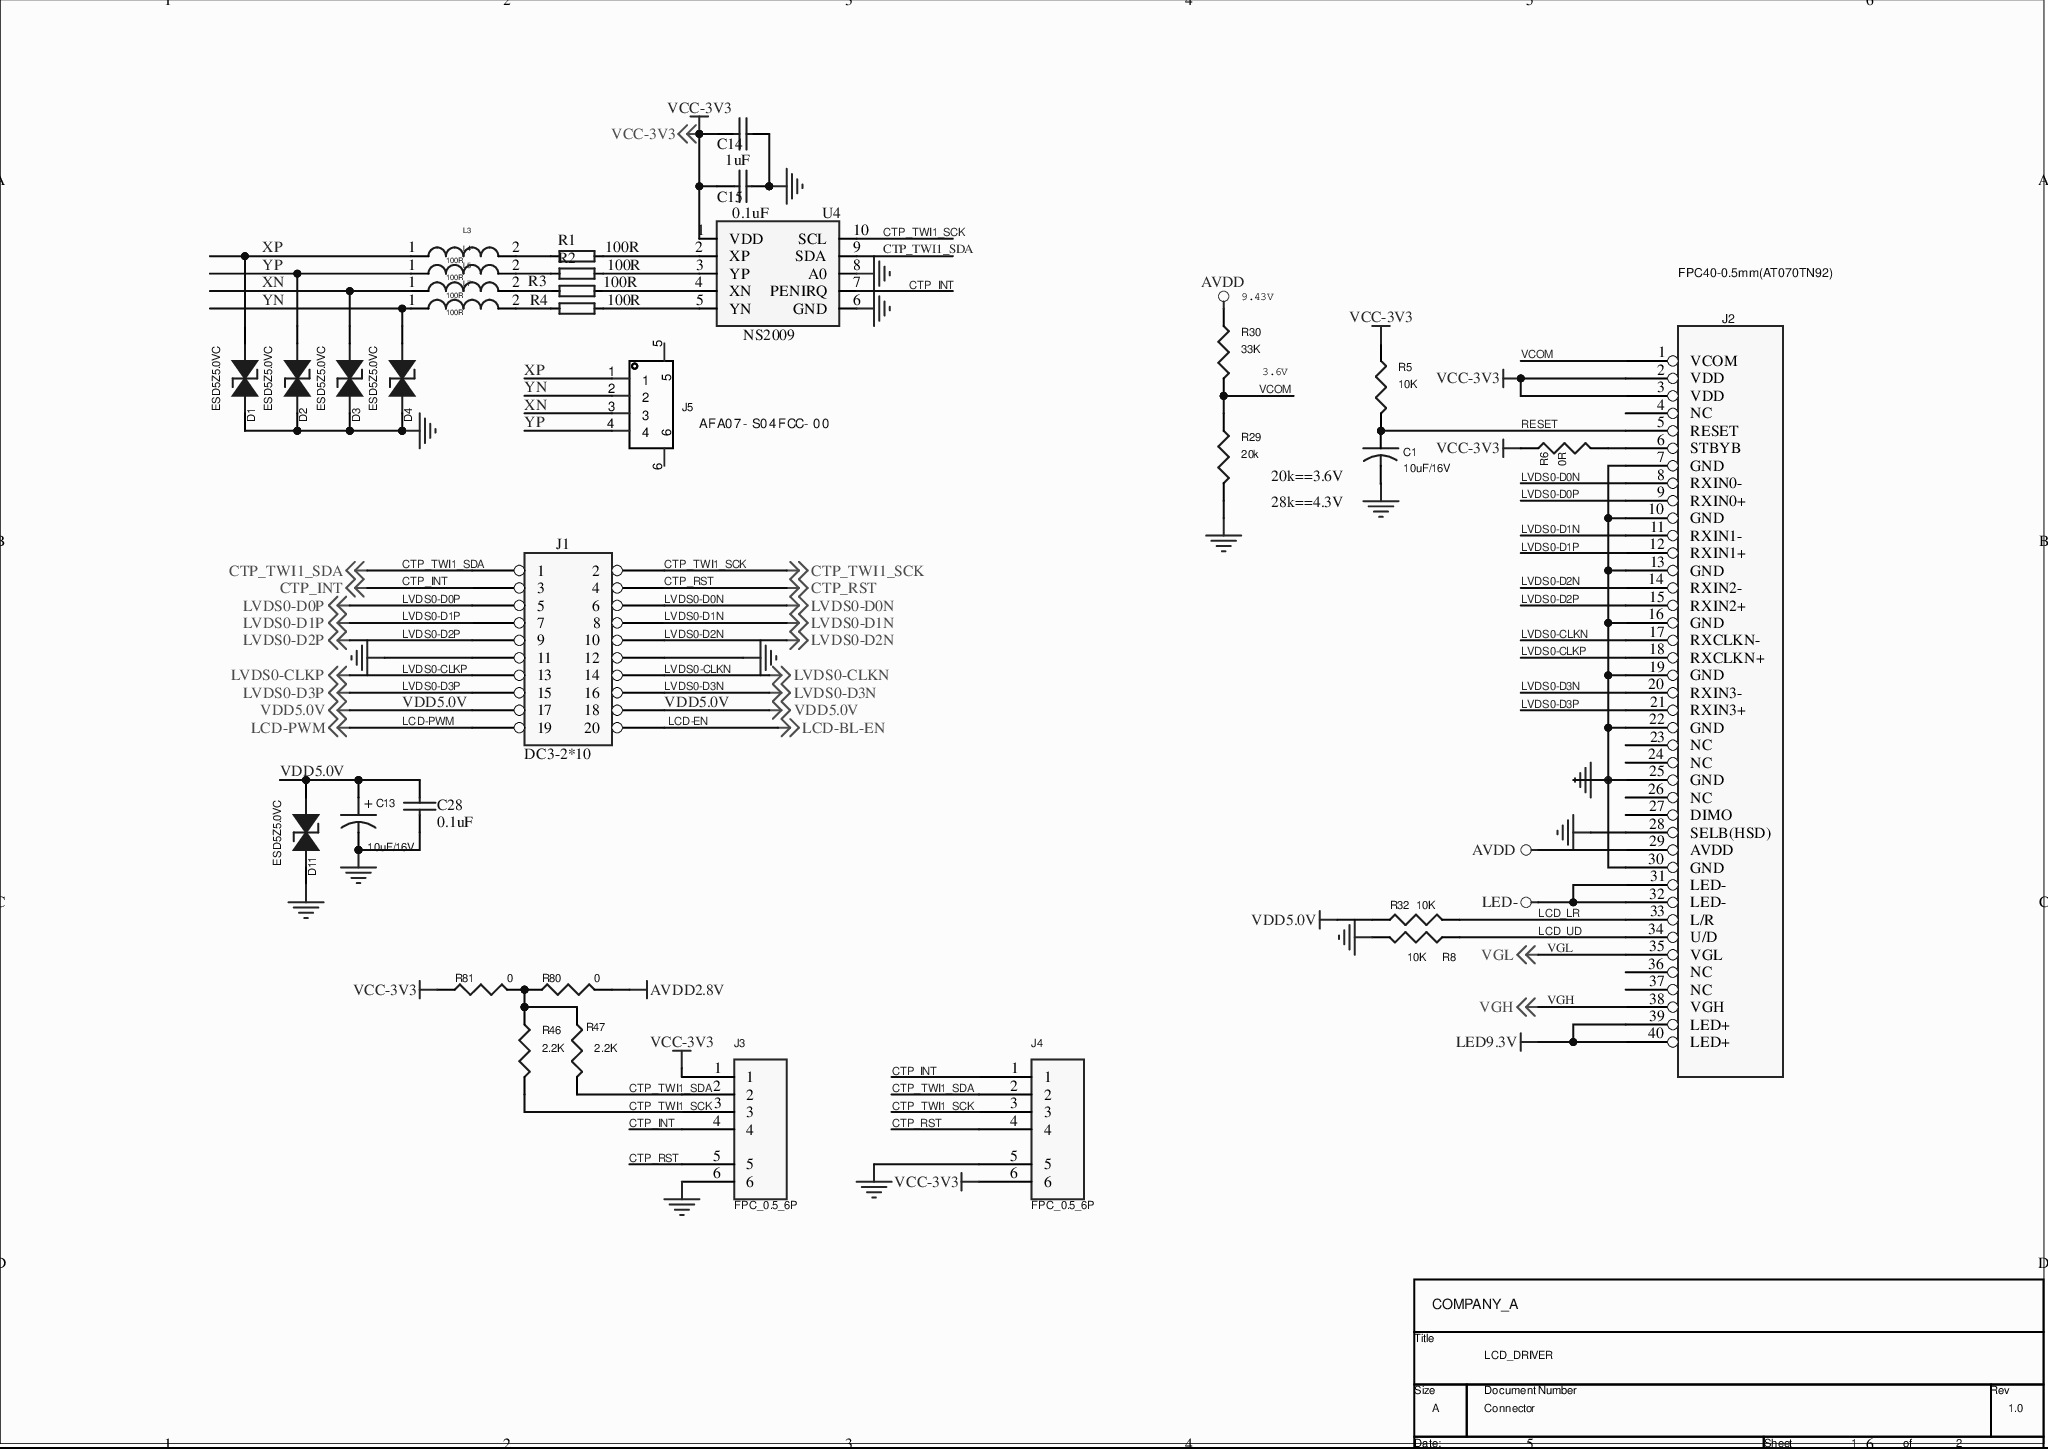
[diagram p0: MISC82162-14.SchDoc]
# Altium project MISC82162-6.PrjPcb
2 sheets, 91 parts. Net scope: global (net labels, ports and power ports of the same name join across sheets).
Board file: MISC82162.PcbDoc
Sheets:
  MISC82162-14.SchDoc
  MISC82162-10.SchDoc

## Sheet MISC82162-14.SchDoc
size 297 x 209 mm

### Parts
*  Page Count: 2  Page Number: 1  Page Size: A  OrgName: COMPANY_A  Title: LCD_DRIVER  RevCode: 1.0  Doc: Connector  (hidden comment: TitleBlock1)  (graphical)
C1  10uF/16V  [0603C]
C13  10uF/16V  [0805C]
C14  1uF  [0603C]
C15  0.1uF  [0603C]
C28  0.1uF  [0603C]
D1  ESD5Z5.0VC  [SOD-523]
D2  ESD5Z5.0VC  [SOD-523]
D3  ESD5Z5.0VC  [SOD-523]
D4  ESD5Z5.0VC  [SOD-523]
D11  ESD5Z5.0VC  [SOD-523]
J1  DC3-2*10  [DC3-2.0-2*10P]
J2  FPC40-0.5mm(AT070TN92)  [FPC40-0.5MM-UP]
J3  FPC_0.5_6P  [FPC_0.5_6P_UP]
J4  FPC_0.5_6P  [FPC_0.5_6P_DOWN]
J5  AFA07-S04FCC-00  [FPC-SMD-1mm4P-RTP]
L3  100R  [0603R]
L4  100R  [0603R]
L5  100R  [0603R]
L7  100R  [0603R]
R1  100R  [0603R]
R2  100R  [0603R]
R3  100R  [0603R]
R4  100R  [0603R]
R5  10K  [0603R]
R6  0R  [0603R]
R8  10K  [0603R]
R29  20k  [0603R]
R30  33K  [0603R]
R32  10K  [0603R]
R46  2.2K  [0603R]
R47  2.2K  [0603R]
R80  0  [0603R]
R81  0  [0603R]
U4  NS2009  [MSOP-10]

### Nets
AVDD: J2.29(AVDD) R30.1
AVDD2.8V: R80.2
GND: C1.2 C13.2 C14.2 C15.2 C28.1 D1.2(CATHODE) D2.2(CATHODE) D3.2(CATHODE) D4.2(CATHODE) D11.2(CATHODE) J1.11 J1.12 J2.7(GND) J2.10(GND) J2.13(GND) J2.16(GND) J2.19(GND) J2.22(GND) J2.25(GND) J2.28(SELB(HSD)) J2.30(GND) J3.6 J4.5 R8.2 R29.2 U4.6(GND) U4.8(A0)
LED9.3V: J2.39(LED+) J2.40(LED+)
LED-: J2.31(LED-) J2.32(LED-)
VCC-3V3: C14.1 C15.1 J2.2(VDD) J2.3(VDD) J3.1 J4.6 R5.1 R6.1 R81.1 U4.1(VDD) ; off-sheet VCC-3V3
VDD5.0V: C13.1 C28.2 D11.1(ANODE) J1.17 J1.18 R32.1 ; off-sheet VDD5.0V
VGH: J2.38(VGH) ; off-sheet VGH
VGL: J2.35(VGL) ; off-sheet VGL
CTP_INT: J1.3 J3.4 J4.1 U4.7(PENIRQ) ; off-sheet CTP_INT
CTP_RST: J1.4 J3.5 J4.4 ; off-sheet CTP_RST
CTP_TWI1_SCK: J1.2 J3.3 J4.3 R46.2 U4.10(SCL) ; off-sheet CTP_TWI1_SCK
CTP_TWI1_SDA: J1.1 J3.2 J4.2 R47.2 U4.9(SDA) ; off-sheet CTP_TWI1_SDA
LCD-BL-EN: J1.20 ; off-sheet LCD-BL-EN  [also labelled LCD-EN]
LCD-PWM: J1.19 ; off-sheet LCD-PWM
LCD_LR: J2.33(L/R) R32.2
LCD_UD: J2.34(U/D) R8.1
LVDS0-CLKN: J1.14 J2.17(RXCLKN-) ; off-sheet LVDS0-CLKN
LVDS0-CLKP: J1.13 J2.18(RXCLKN+) ; off-sheet LVDS0-CLKP
LVDS0-D0N: J1.6 J2.8(RXIN0-) ; off-sheet LVDS0-D0N
LVDS0-D0P: J1.5 J2.9(RXIN0+) ; off-sheet LVDS0-D0P
LVDS0-D1N: J1.8 J2.11(RXIN1-) ; off-sheet LVDS0-D1N
LVDS0-D1P: J1.7 J2.12(RXIN1+) ; off-sheet LVDS0-D1P
LVDS0-D2N: J1.10 J2.14(RXIN2-) ; off-sheet LVDS0-D2N
LVDS0-D2P: J1.9 J2.15(RXIN2+) ; off-sheet LVDS0-D2P
LVDS0-D3N: J1.16 J2.20(RXIN3-) ; off-sheet LVDS0-D3N
LVDS0-D3P: J1.15 J2.21(RXIN3+) ; off-sheet LVDS0-D3P
RESET: C1.1 J2.5(RESET) R5.2
VCOM: J2.1(VCOM) R29.1 R30.2
XN: D3.1(ANODE) J5.3 L5.1
XP: D1.1(ANODE) J5.1 L3.1
YN: D4.1(ANODE) J5.2 L7.1
YP: D2.1(ANODE) J5.4 L4.1
NetJ2_6: J2.6(STBYB) R6.2
NetL3_2: L3.2 R1.1
NetL4_2: L4.2 R2.1
NetL5_2: L5.2 R3.1
NetL7_2: L7.2 R4.1
NetR1_2: R1.2 U4.2(XP)
NetR2_2: R2.2 U4.3(YP)
NetR3_2: R3.2 U4.4(XN)
NetR4_2: R4.2 U4.5(YN)
NetR46_1: R46.1 R47.1 R80.1 R81.2

Not connected (* = marked no-connect by the designer): J2 4(NC) 23(NC) 24(NC) 26(NC) 27(DIMO) 36(NC) 37(NC); J5 5 6

### Notes on the sheet
- (near R30) 9.43V
- (near R30) 3.6V
- 20k==3.6V
- 28k==4.3V

### Library data of the parts
C1 = C
C13 = CAP POL
C14 C15 C28 = CAP: Capacitor
D1-D4 D11 = 1_1.5KE100A: 1ST PART DESCRIPTION: WILL ESD9B5V Bidirection ESD Protection
J2 = HEADER 20X2_3: Populate: YES
J3 J4 = connet_0
J5 = AFC07-S04ECC-00: Manufacturer: JS(钜硕电子); Symbol: FPC 0.5MM 4P Pull type H2.0mm Pick up; Add into BOM: yes; Pitch: 0.5mm; Number of Contacts: 4; Locking Feature: Drawer type; FFC, FCB Thickness: 0.3mm; Name: AFC07-S04ECC-00; Device: AFC07-S04ECC-00; LCSC Part Name: 0.5mm P数:4 抽屉式 上接; Supplier Part: C11082; Manufacturer Part: AFC07-S04ECC-00; Supplier Footprint: SMD,P=0.5mm; JLCPCB Part Class: Extended Part; Supplier: LCSC; Convert to PCB: yes; Mounting Type: Horizontal mount; Contact Type: Top entry; Height Above Board: 2mm
L3-L5 L7 = INDUCTOR
R1 R2 R4 = RES2
R3 = RES2: Designator: R?
R5 R6 R8 R29 R30 R32 R46 R47 R80 R81 = R
* = TitleBlock1: Page Create Date: March  8, 1995

## Sheet MISC82162-10.SchDoc
size A4
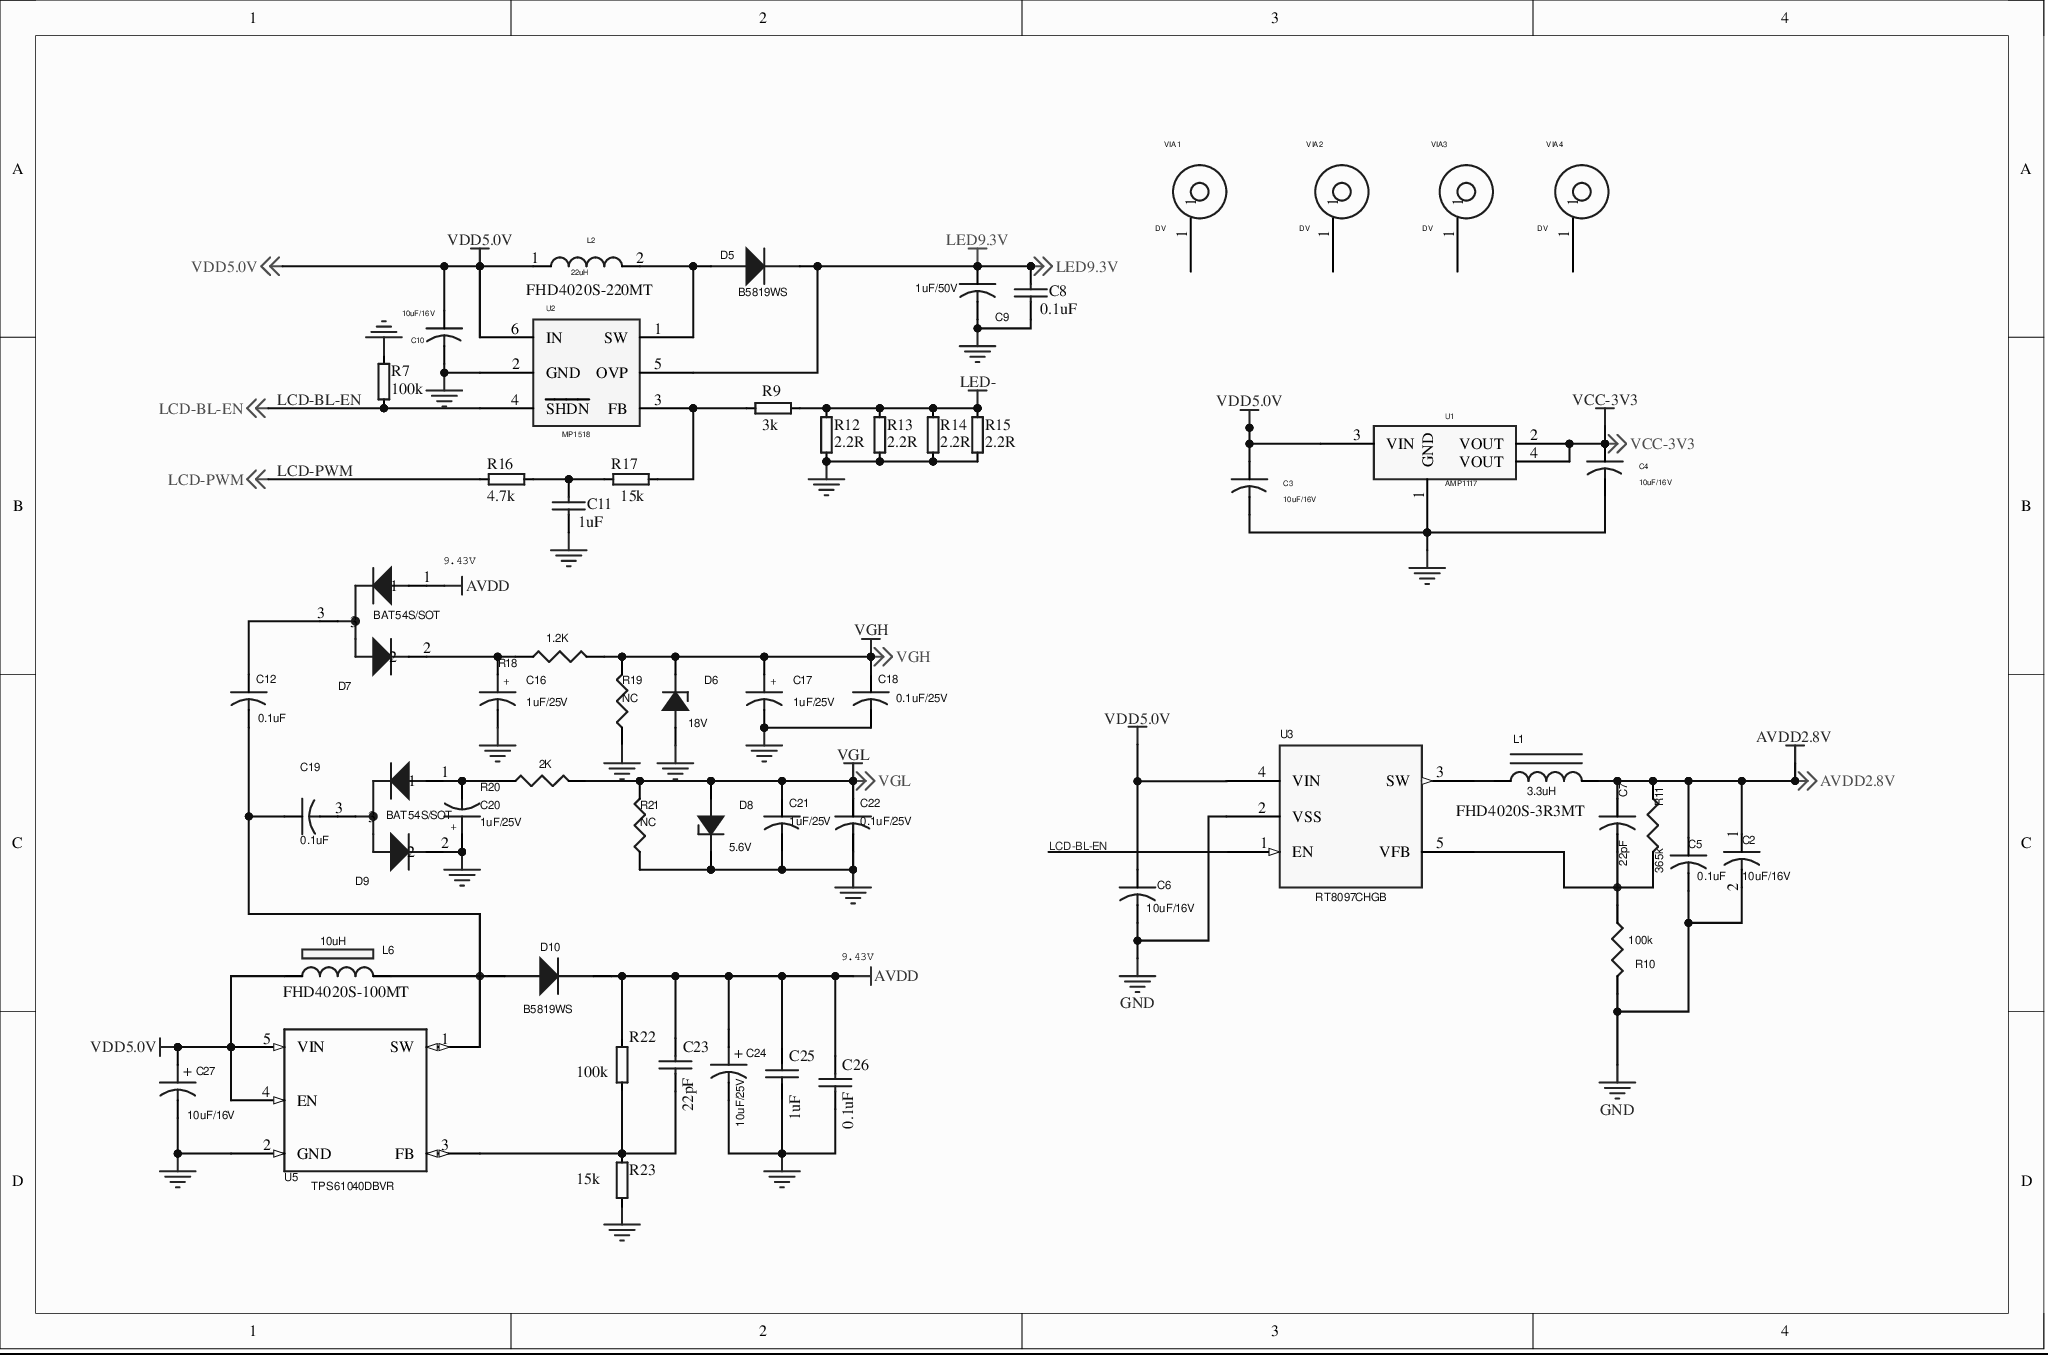
[diagram p1: MISC82162-10.SchDoc]

### Parts
C2  10uF/16V  [0805C]
C3  10uF/16V  [0805C]
C4  10uF/16V  [0805C]
C5  0.1uF  [0603C]
C6  10uF/16V  [0805C]
C7  22pF  [0603C]
C8  0.1uF  [0603C]
C9  1uF/50V  [0603C]
C10  10uF/16V  [0805C]
C11  1uF  [0603C]
C12  0.1uF  [0603C]
C16  1uF/25V  [0805C]
C17  1uF/25V  [0805C]
C18  0.1uF/25V  [0603C]
C19  0.1uF  [0603C]
C20  1uF/25V  [0805C]
C21  1uF/25V  [0603C]
C22  0.1uF/25V  [0603C]
C23  22pF  [0603C]
C24  10uF/25V  [0805C]
C25  1uF  [0603C]
C26  0.1uF  [0603C]
C27  10uF/16V  [0805C]
D5  B5819WS  [SOD-123]
D6  18V  [SOD-123]
D7  BAT54S/SOT  [SOT23]
D8  5.6V  [SOD-123]
D9  BAT54S/SOT  [SOT23]
D10  B5819WS  [SOD-123]
L1  3.3uH  [L-SMD-4*4*1.2]
L2  22uH  [L-SMD-4*4*1.2]
L6  10uH  [L-SMD-4*4*1.2]
R7  100k  [0603R]
R9  3k  [0603R]
R10  100k  [0603C]
R11  365k  [0603R]
R12  2.2R  [0805R]
R13  2.2R  [0805R]
R14  2.2R  [0805R]
R15  2.2R  [0805R]
R16  4.7k  [0603R]
R17  15k  [0603R]
R18  1.2K  [0603R]
R19  NC  [0603R]
R20  2K  [0603R]
R21  NC  [0603R]
R22  100k  [0603R]
R23  15k  [0603R]
U1  AMP1117  [SOT223]
U2  MP1518  [SOT-23-6]
U3  RT8097CHGB  [SOT23-5]
U5  TPS61040DBVR  [SOT-23-5]
VIA1  DV  [M3]
VIA2  DV  [M3]
VIA3  DV  [M3]
VIA4  DV  [M3]

### Nets
AVDD: C23.1 C24.1 C25.1 C26.1 D7.1 D10.2(CATHODE) R22.2
AVDD2.8V: C2.1 C5.1 C7.1 L1.2 R11.1 ; off-sheet AVDD2.8V
GND: C2.2 C3.2 C4.2 C5.2 C6.2 C8.2 C9.2 C10.2 C11.2 C16.2 C17.2 C18.2 C20.1 C21.2 C22.2 C24.2 C25.2 C26.2 C27.2 D6.1(ANODE) D8.2(CATHODE) D9.2 R7.1 R10.2 R12.2 R13.2 R14.2 R15.2 R19.1 R21.1 R23.1 U1.1(GND) U2.2(GND) U3.2(VSS) U5.2(GND)
LED9.3V: C8.1 C9.1 D5.2(CATHODE) U2.5(OVP) ; off-sheet LED9.3V
LED-: R9.1 R12.1 R13.1 R14.1 R15.1
VCC-3V3: C4.1 U1.2(VOUT) U1.4(VOUT) ; off-sheet VCC-3V3
VDD5.0V: C3.1 C6.1 C10.1 C27.1 L2.1 L6.1 U1.3(VIN) U2.6(IN) U3.4(VIN) U5.4(EN) U5.5(VIN) ; off-sheet VDD5.0V
VGH: C17.1 C18.1 D6.2(CATHODE) R18.2 R19.2 ; off-sheet VGH
VGL: C21.1 C22.1 D8.1(ANODE) R20.2 R21.2 ; off-sheet VGL
LCD-BL-EN: R7.2 U2.4(~{SHDN}) U3.1(EN) ; off-sheet LCD-BL-EN
LCD-PWM: R16.2 ; off-sheet LCD-PWM
NetC7_2: C7.2 R10.1 R11.2 U3.5(VFB)
NetC11_1: C11.1 R16.1 R17.2
NetC12_1: C12.1 D7.3
NetC12_2: C12.2 C19.1 D10.1(ANODE) L6.2 U5.1(SW)
NetC16_1: C16.1 D7.2 R18.1
NetC19_2: C19.2 D9.3
NetC20_2: C20.2 D9.1 R20.1
NetC23_2: C23.2 R22.1 R23.2 U5.3(FB)
NetD5_1: D5.1(ANODE) L2.2 U2.1(SW)
NetL1_1: L1.1 U3.3(SW)
NetR9_2: R9.2 R17.1 U2.3(FB)

Not connected (* = marked no-connect by the designer): VIA1 1; VIA2 1; VIA3 1; VIA4 1

### Notes on the sheet
- (near L2) FHD4020S-220MT
- (near D7) 9.43V
- FHD4020S-3R3MT
- (near L6) FHD4020S-100MT
- 9.43V

### Library data of the parts
C2 = CAPACITOR_0
C3 C4 C10 C12 C18 C19 C21 C22 = C
C5-C7 = CAPACITOR
C8 C11 C23 C25 C26 = CAP: Capacitor
C9 = C_Dup1
C16 C17 C20 C24 C27 = CAP POL
D5 D10 = BAS21/SOT_1
D6 D8 = DIODE BREAKDOWN_1
L1 = INDUCTOR IRON
L2 = INDUCTOR
L6 = CHOKE TORROID-FERRITE
R7 R9 R12-R17 R22 R23 = RES2
R10 R11 = R
R18-R21 = RESISTOR
U1 = LM7805/TO_6
U2 = PT4110_0
U3 = XC9235_0
U5 = X9C102/SO_2
VIA1-VIA4 = DV_0

## Nets that join several sheets
AVDD: MISC82162-14 (J2.29 R30.1), MISC82162-10 (7 pins)
AVDD2.8V: MISC82162-14 (R80.2), MISC82162-10 (5 pins)
GND: MISC82162-14 (27 pins), MISC82162-10 (35 pins)
LED9.3V: MISC82162-14 (J2.39 J2.40), MISC82162-10 (C8.1 C9.1 D5.2 U2.5)
LED-: MISC82162-14 (J2.31 J2.32), MISC82162-10 (5 pins)
VCC-3V3: MISC82162-14 (10 pins), MISC82162-10 (C4.1 U1.2 U1.4)
VDD5.0V: MISC82162-14 (6 pins), MISC82162-10 (11 pins)
VGH: MISC82162-14 (J2.38), MISC82162-10 (5 pins)
VGL: MISC82162-14 (J2.35), MISC82162-10 (5 pins)
LCD-BL-EN: MISC82162-14 (J1.20), MISC82162-10 (R7.2 U2.4 U3.1)
LCD-PWM: MISC82162-14 (J1.19), MISC82162-10 (R16.2)